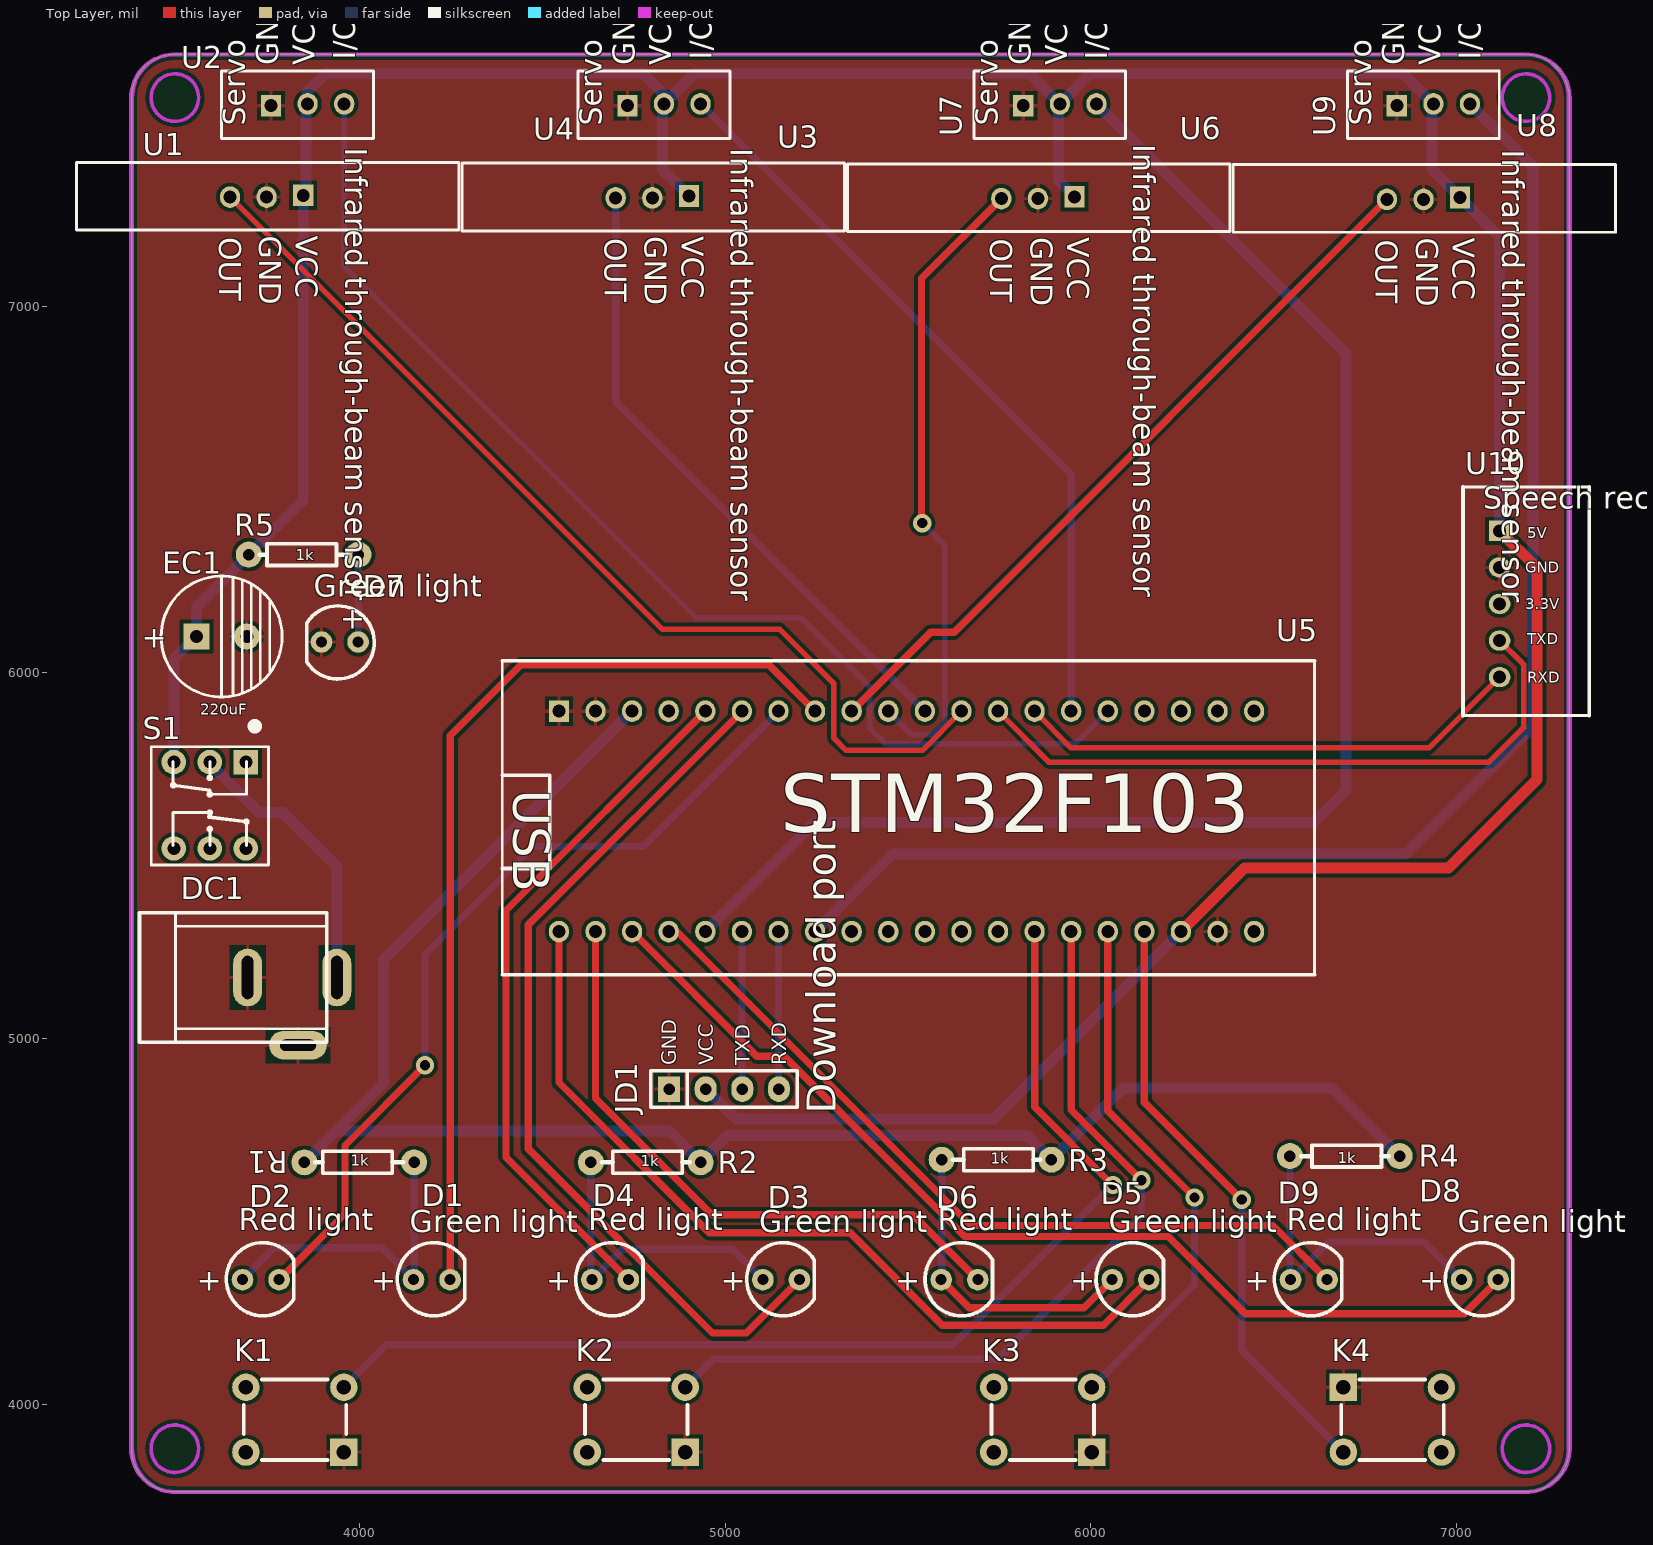
[diagram p0: Top Layer view]
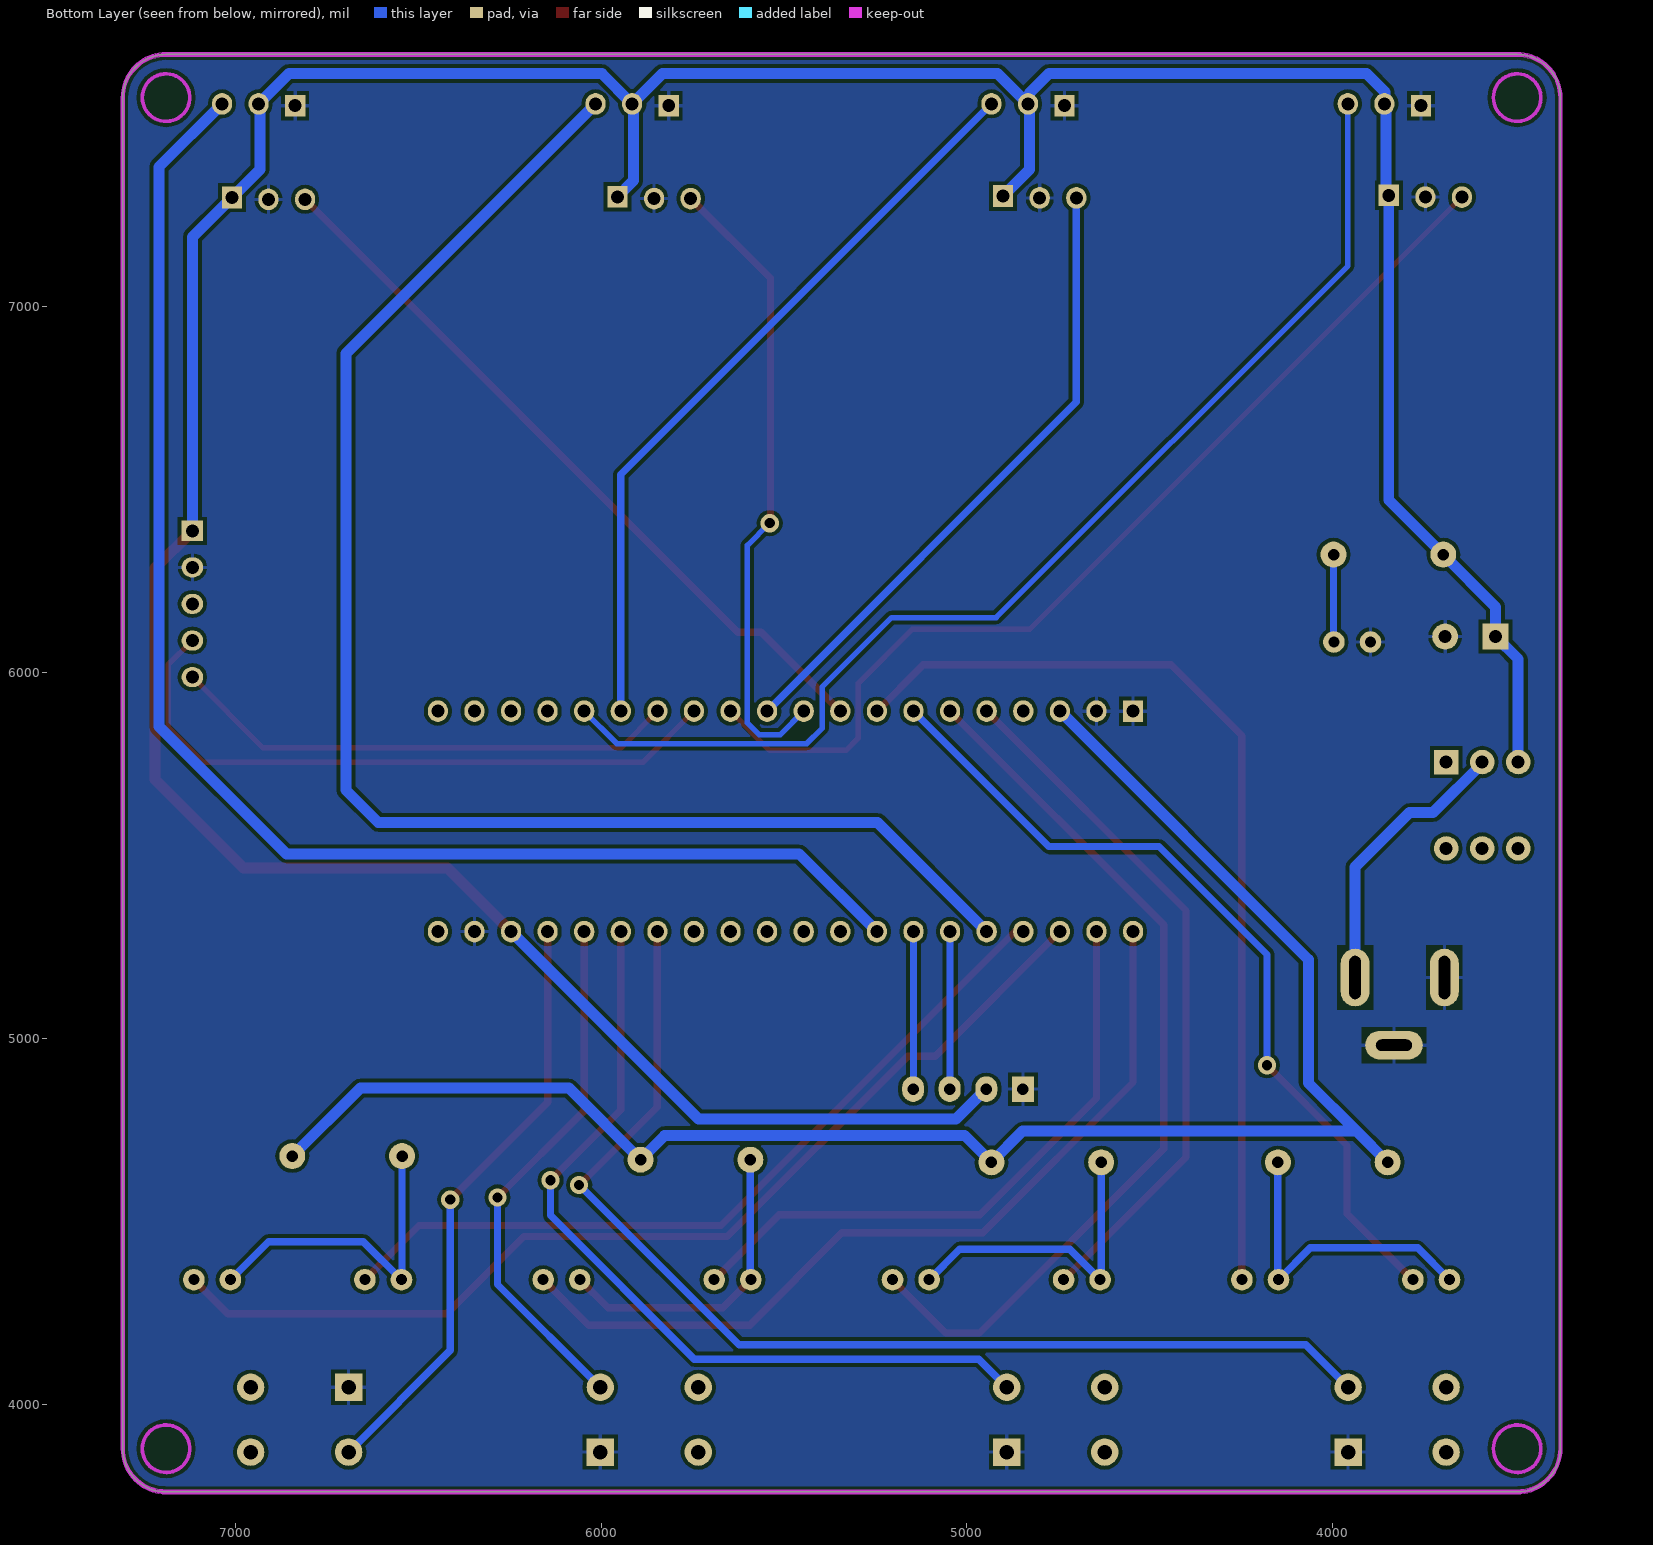
[diagram p1: Bottom Layer view, seen from below]
# Altium PCB MISC49886.pcbdoc
Units mil, origin at the board's own origin, x right, y up, seen from the top; angles counter-clockwise.
Board outline 3929.13 x 3929.13 mil, 2 copper layers (Top Layer, Bottom Layer); 32 components, 43 nets, 128 pads, 6 vias.

## Layer stack, top to bottom (the 12.6 mil dielectric is the usual default, probably not edited)
Top Solder Mask Layer: solder mask 1.4, FR-4, Dk 4.8
Top Layer: signal copper 1.4
Substrate1: surface 12.6, FR-4, Dk 4.8
Bottom Layer: signal copper 1.4
Bottom Solder Mask Layer: solder mask 1.4, FR-4, Dk 4.8

## Board outline
3378,7572.02 3378,3879.11 ccw(c3496.11,3879.11) 3496.11,3761 7189.02,3761 ccw(c7189.02,3879.11) 7307.13,3879.11 7307.13,7572.02 ccw(c7189.02,7572.02) 7189.02,7690.13 3496.11,7690.13 ccw(c3496.11,7572.02)

## Design rules (kind name [scope] priority, off if disabled: settings)
BoardOutlineClearance Clearance_1 [All] p2: genericclearance=10 ignorepadtopadclearanceinfootprint=FALSE except(0: Arc-SplitContinuation Track-SplitContinuation SMDPad-SplitContinuation THPad-SplitContinuation Via-SplitContinuation Fill-SplitContinuation Region-SplitContinuation Poly-SplitContinuation Text-SplitContinuation Hole-SplitContinuation; 6: SMDPad-CutoutEdge THPad-CutoutEdge Via-CutoutEdge Fill-CutoutEdge Region-CutoutEdge Text-CutoutEdge; 6.9: Hole-CutoutEdge; 10: Arc-OutlineEdge Track-OutlineEdge SMDPad-OutlineEdge THPad-OutlineEdge Via-OutlineEdge Fill-OutlineEdge Region-OutlineEdge Poly-OutlineEdge Text-OutlineEdge Hole-OutlineEdge Poly-CutoutEdge; 11.8: Arc-CutoutEdge Track-CutoutEdge)
Clearance [All] p1: gap=10 ignorepadtopadclearanceinfootprint=FALSE
DiffPairsRouting [All] p1: maxlimit=10 minlimit=6 mostfreqgap=6 toplayer_minwidth=0 toplayer_prefwidth=0 toplayer_maxwidth=0 toplayer_mingap=10 toplayer_prefgap=10 toplayer_maxgap=10 bottomlayer_minwidth=0 bottomlayer_prefwidth=0 bottomlayer_maxwidth=0 bottomlayer_mingap=10 bottomlayer_prefgap=10 bottomlayer_maxgap=10 maxuncoupledlength=10
HoleToHoleClearance ComponentClearance [All] p1: gap=10 allowstackedmicrovias=TRUE
Length netLength [All] p1: minlimit=0 maxlimit=0
MatchedLengths netLengthTolerance [All] p1: tolerance=1000
PolygonConnect [All] p1: connectstyle=Relief reliefconductorwidth=10 reliefentries=4 polygonreliefangle="90 Angle" airgapwidth=10 via.connectstyle=Relief via.reliefconductorwidth=10 via.reliefentries=4 via.polygonreliefangle="90 Angle" via.airgapwidth=10
RoutingVias [All] p1: holewidth=28 width=50 viastyle="Through Hole" minholewidth=28 minwidth=50 maxholewidth=28 maxwidth=50
SolderMaskExpansion [All] p1: expansion=4 istentingtop=FALSE
Width [All] p1: maxlimit=10 minlimit=10 preferedwidth=10 toplayer_minwidth=10 toplayer_maxwidth=40 toplayer_prefwidth=20 bottomlayer_minwidth=10 bottomlayer_maxwidth=40 bottomlayer_prefwidth=20
2 further rules are at their usual default settings.

## Components (designator, comment, footprint, x,y, rotation, side; value= is the part's Value field where it differs from the comment)
D1 "LED" LED5-GRE 4198.43,4341 r0 top
D2 "LED" LED5-RED 3731,4341 r0 top
D3 "LED" LED5-GRE 5153.29,4341 r0 top
D4 "LED" LED5-RED 4685.86,4341 r0 top
D5 "LED" LED5-GRE 6108.14,4341 r0 top
D6 "LED" LED5-RED 5640.71,4341 r0 top
D7 "LED" LED5-GRE 3947,6084 r180 top
D8 "LED" LED5-GRE 7063,4341 r0 top
D9 "LED" LED5-RED 6595.57,4341 r0 top
DC1 "DC_Socket" DC-005 3939,5167 r180 top
EC1 "220uF" DIP-EC3.5X8X11.5 3555,6099 r0 top
JD1 "Download port" 下载口 5187,5082 r180 top
K1 "BUTTOM" DIP-6X6X5 3958,3869.83 r180 top
K2 "BUTTOM" DIP-6X6X5 4891,3869.83 r180 top
K3 "BUTTOM" DIP-6X6X5 6002,3869.83 r180 top
K4 "BUTTOM" DIP-6X6X5 6690,4047 r0 top
R1 "1k" AXIAL0.3-1k 4150,4662 r180 top
R2 "1K" AXIAL0.3-1k 4633,4662 r0 top
R3 "1k" AXIAL0.3-1k 5592,4669 r0 top
R4 "1k" AXIAL0.3-1k 6544,4679 r0 top
R5 "1k" AXIAL0.3-1k 3998,6323 r180 top
S1 "KFT DIP-8X8" "KFT DIP-8X8" 3430,5801 r270 top
U1 "JS" JS 3217,7400 r270 top
U2 "SG90" SG90 4149,7460 r90 top
U3 "JS" JS 4271,7398 r270 top
U4 "SG90" SG90 5123,7460 r90 top
U5 "STM32F103" STM32F103 4546,5895 r270 top
U6 "JS" JS 5325,7396 r270 top
U7 "SG90" SG90 6205,7460 r90 top
U8 "JS" JS 6379,7394 r270 top
U9 "SG90" SG90 7226,7460 r90 top
U10 "SNR8016" SNR8016 7012,5878 r0 top

## Footprints (in the part's own frame and the unit in brackets; to place one, negate y for a bottom-side part, rotate by r counter-clockwise, add the part's x,y. Pads: shape width x height; smd on the part's side, far side on the other; paste and mask are expansions set on the pad)
AXIAL0.3-1k [mm]
  round 1.8 hole 0.8: 1(0,0) 2(7.62,0)
  silkscreen extent 0.76,-0.76 6.86,0.76
DC-005 [mm]
  oval 2x4 hole 0.8 slot 3 at 90 deg: 1(0,0) 2(6.2,0)
  oval 4x2 hole 0.8 slot 2.5 at 0 deg: 3(2.7,4.7)
  silkscreen extent 0.72,-4.5 13.7,4.5
DIP-6X6X5 [mm]
  rect 1.9x1.9 hole 1: 1(0,0)
  round 1.9 hole 1: 2(0,-4.5) 3(6.8,-4.5) 4(6.8,0)
  silkscreen extent -0.16,-5.04 6.96,0.54
DIP-EC3.5X8X11.5 [mm]
  rect 1.8x1.8 hole 0.9: 1(0,0)
  round 1.8 hole 0.9: 2(3.5,0)
  silkscreen extent -2.45,-4.2 5.95,4.2
JS [mm]
  rect 1.5x1.4 hole 0.9: 1(2.413,16.002)
  oval 1.5x1.4 hole 0.9: 2(2.54,13.462) 3(2.54,10.922)
  silkscreen extent 0.13,0.25 4.83,26.8
"KFT DIP-8X8" [mm]
  rect 1.7x1.7 hole 0.9: 1(1.143,6.604)
  round 1.7 hole 0.9: 2(1.143,4.104) 3(1.143,1.604) 4(7.143,1.604) 5(7.143,4.104) 6(7.143,6.604)
  silkscreen extent -1.54,0.04 8.3,8.17
LED5-GRE [mm]
  round 1.5 hole 0.762: A(-1.27,0) K(1.27,0)
  silkscreen extent -2.39,-2.51 2.29,2.57
LED5-RED [mm]
  round 1.5 hole 0.762: A(-1.27,0) K(1.27,0)
  silkscreen extent -2.39,-2.51 2.29,2.57
SG90 [mm]
  rect 1.5x1.4 hole 0.9: 1(2.286,9.906)
  oval 1.5x1.4 hole 0.9: 2(2.413,7.366) 3(2.413,4.826)
  silkscreen extent 0,2.79 4.7,13.33
SNR8016 [mm]
  rect 1.5x1.4 hole 0.9: 1(2.667,12.954)
  oval 1.5x1.4 hole 0.9: 2(2.667,10.414) 3(2.667,7.874) 4(2.667,5.334) 5(2.667,2.794)
  silkscreen extent 0.13,0.13 8.89,16
STM32F103 [mm]
  rect 1.5x1.4 hole 0.9: 1(0,0)
  oval 1.5x1.4 hole 0.9: 2(0,2.54) 3(0,5.08) 4(0,7.62) 5(0,10.16) 6(0,12.7) 7(0,15.24) 8(0,17.78) 9(0,20.32) 10(0,22.86) 11(0,25.4) 12(0,27.94) 13(0,30.48) 14(0,33.02) 15(0,35.56) 16(0,38.1) 17(0,40.64) 18(0,43.18) 19(0,45.72) 20(0,48.26) 25(15.3,48.26) 26(15.3,45.72) 27(15.3,43.18) 28(15.3,40.64) 29(15.3,38.1) 30(15.3,35.56) 31(15.3,33.02) 32(15.3,30.48) 33(15.3,27.94) 34(15.3,25.4) 35(15.3,22.86) 36(15.3,20.32) 37(15.3,17.78) 38(15.3,15.24) 39(15.3,12.7) 40(15.3,10.16) 41(15.3,7.62) 42(15.3,5.08) 43(15.3,2.54) 44(15.3,0)
  silkscreen extent -3.5,-3.94 18.29,52.45
下载口 [mil]
  rect 60x70 hole 32: 1(340,220)
  oval 60x70 hole 32: 2(240,220) 3(140,220) 4(40,220)
  silkscreen extent -10,170 390,270

## Via types
v1: diameter 50, hole 28, Top Layer to Bottom Layer, 6 vias

## Nets (pads, with @x,y where several pads share a name; then routed paths per layer and width w, separated by ;. In a path a pad name is that pad's centre, name@x,y a point inside that pad or via, vN(x,y) a via of type N, cw(c..) or ccw(c..) an arc to the next point about the centre after c; other vN are vias at no path point)
GND: D7.K DC1.2 DC1.3 EC1.2 JD1.1 K1.1 K2.1 K3.1 K4.1 U1.2 U2.1 U3.2 U4.1 U5.1 U5.2 U5.26 U6.2 U7.1 U8.2 U9.1 U10.2
NetD1_A: D1.A D2.A R1.1 | length 858.9
  Bottom Layer w20: D2.A 3768,4428 4061.43,4428 D1.A ; D1.A@4150,4342.57 R1.1
NetD3_A: D3.A D4.A R2.1 | length 858.4
  Bottom Layer w20: R2.1 4633,4343.86 D4.A 4718.86,4424 5020.29,4424 D3.A
NetD5_A: D5.A D6.A R3.1 | length 859.8
  Top Layer w20: D6.A 5667.71,4264 5981.14,4264 D5.A
  Bottom Layer w20: D6.A 5592,4342.29 R3.1
NetD7_A: D7.A R5.1 | length 238
  Bottom Layer w20: D7.A@3998,6085 R5.1
NetD8_A: D8.A D9.A R4.1 | length 890
  Bottom Layer w20: D9.A@6544,4342.57 R4.1 ; D9.A 6649.57,4445 6909,4445 D8.A
NetDC1_1: DC1.1 S1.2 | length 770.6
  Bottom Layer w30: S1.2 3591.57,5752.14 3725.72,5618 3790,5618 3939,5469 DC1.1
PA0: U2.3 U5.16 | length 3174
  Bottom Layer w15: U2.3 3959,7112 4920,6151 5206,6151 5396,5961 5396,5848 5438,5806 5957,5806 U5.16
PA1: U4.3 U5.15 | length 2079.6
  Bottom Layer w20: U4.3 5946,6542 U5.15
PA2: U5.14 U10.5 | length 1392.4
  Top Layer w15: U5.14 5946,5795 6924,5795 U10.5
PA3: U5.13 U10.4 | length 1799.1
  Top Layer w15: U5.13 5886,5755 7087,5755 7183,5851 7183,6022 U10.4
PA4: U1.3 U5.12 | length 2756.9
  Top Layer w15: U1.3 4828,6119 5149,6119 5297,5971 5297,5822 5331,5788 5539,5788 U5.12
PA5: U3.3 U5.11 | length 1753
  Bottom Layer w20: U3.3 4701,6740 U5.11
PA6: U5.10 U6.3 | length 1744.3
  Top Layer w20: v1@5537,6407 5537,7078 U6.3
  Bottom Layer w15: U5.10 5510,5831 5568,5831 5600,5863 5600,6348 v1(5539,6409)
PA7: U5.9 U8.3 | length 2042.5
  Top Layer w20: U5.9 5562,6111 5626,6111 U8.3
PA8: U5.40 U7.3 | length 4069.5
  Bottom Layer w30: U5.40 5244.36,5591 6609,5591 6697,5679 6697,6873 U7.3
PA9: JD1.3 U5.39 | length 429.6
  Bottom Layer w20: JD1.3@5046,4863 U5.39
PA10: JD1.4 U5.38 | length 429.6
  Bottom Layer w20: JD1.4@5146,4863 U5.38
PA11: U5.37 U9.3 | length 3967.4
  Bottom Layer w30: U5.37 5458.36,5505 6860,5505 7208,5853 7208,7383 U9.3
PA12: U5.36
PA15: U5.35
PB0: D1.K U5.8 | length 2617.8
  Top Layer w20: D1.K 4248.43,5828.43 4442,6022 5119,6022 U5.8
PB1: D2.K U5.7 | length 2295.7
  Top Layer w20: D2.K 3961,4521 3961,4708 v1(4180,4927)
  Bottom Layer w20: v1(4180,4927) 4180,5230 4475,5525 4776,5525 U5.7
PB3: U5.34
PB4: U5.33
PB5: U5.32
PB6: K1.2 U5.31 | length 3102
  Top Layer w20: U5.31 5846,4813 v1@6052,4607
  Bottom Layer w20: K1.2 4074,4163 5623,4163 v1(6060,4600)
PB7: K2.2 U5.30 | length 2296.8
  Top Layer w20: U5.30 5946,4805 v1(6138,4613)
  Bottom Layer w20: K2.2 4968,4124 5745,4124 6138,4517 v1(6138,4613)
PB8: K3.2 U5.29 | length 1460.2
  Top Layer w20: U5.29 6046,4803 v1(6283,4566)
  Bottom Layer w20: K3.2 6283,4328 v1(6283,4566)
PB9: K4.2 U5.28 | length 1648.1
  Top Layer w20: U5.28 6146,4826 v1(6412,4560)
  Bottom Layer w20: v1(6412,4560) 6412,4147.83 K4.2
PB10: D3.K U5.6 | length 2448.2
  Top Layer w20: U5.6 4462,5311 4462,4699 4965.71,4195.29 5057.57,4195.29 D3.K
PB11: D4.K U5.5 | length 1918.4
  Top Layer w20: D4.K 4401,4675.86 4401,5350 U5.5
PB12: D5.K U5.44 | length 2350.8
  Top Layer w20: U5.44 4546,4880 4957,4469 5342,4469 5594,4217 6034.14,4217 D5.K
PB13: D6.K U5.43 | length 1705.8
  Top Layer w20: U5.43 4646,4837 4964,4519 5512.71,4519 D6.K
PB14: D8.K U5.42 | length 2838.2
  Top Layer w20: U5.42 5086.64,4952 5162,4952 5655,4459 6211,4459 6422,4248 7020,4248 D8.K
PB15: D9.K U5.41 | length 2193.8
  Top Layer w20: U5.41 4868.36,5292.64 5672,4489 6497.57,4489 D9.K
PC13: U5.19
PC14: U5.18
PC15: U5.17
R: U5.4
VB: U5.20
VCC: EC1.1 JD1.2 R5.2 S1.3 U1.1 U2.2 U3.1 U4.2 U5.27 U6.1 U7.2 U8.1 U9.2 U10.1 | length 10465.3
  Top Layer w30: U5.27 6419.36,5466 6977,5466 7219,5708 7219,6286 U10.1
  Bottom Layer w30: S1.3 3493.15,6037.15 EC1.1 3555,6180 R5.2 3847,6472 U1.1 3855,7313 3855,7564 3857,7566 3857,7587 3908,7638 4776,7638 4829,7585 4829,7375 U3.1 ; U4.2 4916,7638 5832,7638 U7.2 5998,7638 6853,7638 U9.2 ; JD1.2@4956,4854 5030,4780 5733.36,4780 U5.27 ; U7.2@5911,7555 5911,7345 U6.1 ; U9.2@6932,7555 6932,7376 U8.1 7117,7191 U10.1
VCC_3V3: R1.2 R2.2 R3.2 R4.2 U5.3 | length 4764.1
  Bottom Layer w30: R1.2 3935,4747 ; U5.3 4067,5216 4067,4879 3935,4747 ; R4.2 6658,4865 6088,4865 R3.2 5826,4735 5006,4735 R2.2 4848,4747 3935,4747
pads on no net: K1.3 K1.4 K2.3 K2.4 K3.3 K3.4 K4.3 K4.4 S1.1 S1.4 S1.5 S1.6 U5.25 U10.3

## Polygon pours and split planes (outlines as drawn)
GND on Bottom Layer (solid, remove dead copper, pour order 6): 3000,7913 3018,7931 7474,7931 7474,3375 7367,3268 7161,3474 3053,3474
GND on Top Layer (solid, remove dead copper, pour order 8): 3089,7743 7582,7743 7456,7617 7456,3000 3715,3000 3250,3465

## Keep-outs
Board Outline Layer:
  region: 7312.13,3879.11 7311.75,3869.45 7310.62,3859.85 7308.73,3850.37 7306.11,3841.07 7302.76,3832 7298.72,3823.22 7293.99,3814.79 7288.62,3806.75 7282.64,3799.16 7276.08,3792.06 7268.98,3785.5 7261.39,3779.51 7253.35,3774.14 7244.91,3769.42 7236.14,3765.37 7227.07,3762.03 7217.76,3759.4 7208.28,3757.52 7198.68,3756.38 7189.02,3756 7187.11,3756.38 7185.49,3757.46 7184.4,3759.09 7184.02,3761 7184.4,3762.91 7185.49,3764.54 7187.11,3765.62 7189.02,3766 7198.36,3766.39 7207.64,3767.54 7216.79,3769.46 7225.75,3772.13 7234.46,3775.53 7242.86,3779.63 7250.89,3784.42 7258.5,3789.85 7265.63,3795.89 7272.24,3802.5 7278.28,3809.64 7283.72,3817.24 7288.5,3825.28 7292.61,3833.67 7296.01,3842.38 7298.67,3851.34 7300.59,3860.49 7301.75,3869.77 7302.13,3879.11 7302.51,3881.02 7303.6,3882.65 7305.22,3883.73 7307.13,3884.11 7309.05,3883.73 7310.67,3882.65 7311.75,3881.02
  region: 7312.13,7572.02 7311.75,7570.11 7310.67,7568.49 7309.05,7567.4 7307.13,7567.02 7305.22,7567.4 7303.6,7568.49 7302.51,7570.11 7302.13,7572.02 7301.75,7581.36 7300.59,7590.64 7298.67,7599.79 7296.01,7608.75 7292.61,7617.46 7288.5,7625.86 7283.72,7633.89 7278.28,7641.5 7272.24,7648.63 7265.63,7655.24 7258.5,7661.28 7250.89,7666.72 7242.86,7671.5 7234.46,7675.61 7225.75,7679.01 7216.79,7681.67 7207.64,7683.59 7198.36,7684.75 7189.02,7685.13 7187.11,7685.51 7185.49,7686.6 7184.4,7688.22 7184.02,7690.13 7184.4,7692.05 7185.49,7693.67 7187.11,7694.75 7189.02,7695.13 7198.68,7694.75 7208.28,7693.62 7217.76,7691.73 7227.07,7689.11 7236.14,7685.76 7244.91,7681.72 7253.35,7676.99 7261.39,7671.62 7268.98,7665.64 7276.08,7659.08 7282.64,7651.98 7288.62,7644.39 7293.99,7636.35 7298.72,7627.91 7302.76,7619.14 7306.11,7610.07 7308.73,7600.76 7310.62,7591.28 7311.75,7581.68
  region: 3383,7572.02 3382.62,7570.11 3381.54,7568.49 3379.91,7567.4 3378,7567.02 3376.09,7567.4 3374.46,7568.49 3373.38,7570.11 3373,7572.02 3373.38,7581.68 3374.52,7591.28 3376.4,7600.76 3379.03,7610.07 3382.37,7619.14 3386.42,7627.91 3391.14,7636.35 3396.51,7644.39 3402.5,7651.98 3409.06,7659.08 3416.16,7665.64 3423.75,7671.62 3431.79,7676.99 3440.22,7681.72 3449,7685.76 3458.07,7689.11 3467.37,7691.73 3476.85,7693.62 3486.45,7694.75 3496.11,7695.13 3498.02,7694.75 3499.65,7693.67 3500.73,7692.05 3501.11,7690.13 3500.73,7688.22 3499.65,7686.6 3498.02,7685.51 3496.11,7685.13 3486.77,7684.75 3477.49,7683.59 3468.34,7681.67 3459.38,7679.01 3450.67,7675.61 3442.28,7671.5 3434.24,7666.72 3426.64,7661.28 3419.5,7655.24 3412.89,7648.63 3406.85,7641.5 3401.42,7633.89 3396.63,7625.86 3392.53,7617.46 3389.13,7608.75 3386.46,7599.79 3384.54,7590.64 3383.39,7581.36
  region: 3496.11,3756 3486.45,3756.38 3476.85,3757.52 3467.37,3759.4 3458.07,3762.03 3449,3765.37 3440.22,3769.42 3431.79,3774.14 3423.75,3779.51 3416.16,3785.5 3409.06,3792.06 3402.5,3799.16 3396.51,3806.75 3391.14,3814.79 3386.42,3823.22 3382.37,3832 3379.03,3841.07 3376.4,3850.37 3374.52,3859.85 3373.38,3869.45 3373,3879.11 3373.38,3881.02 3374.46,3882.65 3376.09,3883.73 3378,3884.11 3379.91,3883.73 3381.54,3882.65 3382.62,3881.02 3383,3879.11 3383.39,3869.77 3384.54,3860.49 3386.46,3851.34 3389.13,3842.38 3392.53,3833.67 3396.63,3825.28 3401.42,3817.24 3406.85,3809.64 3412.89,3802.5 3419.5,3795.89 3426.64,3789.85 3434.24,3784.42 3442.28,3779.63 3450.67,3775.53 3459.38,3772.13 3468.34,3769.46 3477.49,3767.54 3486.77,3766.39 3496.11,3766 3498.02,3765.62 3499.65,3764.54 3500.73,3762.91 3501.11,3761 3500.73,3759.09 3499.65,3757.46 3498.02,3756.38
  region: 3561.07,3879.11 cw(c3496.11,3879.11) 3431.15,3879.11 cw(c3496.11,3879.11)
  circle w10: c3496.11,3879.11 r64.96
  region: 7253.98,3879.11 cw(c7189.02,3879.11) 7124.06,3879.11 cw(c7189.02,3879.11)
  circle w10: c7189.02,3879.11 r64.96
  region: 7253.98,7572.02 cw(c7189.02,7572.02) 7124.06,7572.02 cw(c7189.02,7572.02)
  circle w10: c7189.02,7572.02 r64.96
  region: 3561.07,7572.02 cw(c3496.11,7572.02) 3431.15,7572.02 cw(c3496.11,7572.02)
  circle w10: c3496.11,7572.02 r64.96
  region: 7194.02,3761 7193.64,3759.09 7192.56,3757.46 7190.94,3756.38 7189.02,3756 3496.11,3756 3494.2,3756.38 3492.57,3757.46 3491.49,3759.09 3491.11,3761 3491.49,3762.91 3492.57,3764.54 3494.2,3765.62 3496.11,3766 7189.02,3766 7190.94,3765.62 7192.56,3764.54 7193.64,3762.91
  region: 7194.02,7690.13 7193.64,7688.22 7192.56,7686.6 7190.94,7685.51 7189.02,7685.13 3496.11,7685.13 3494.2,7685.51 3492.57,7686.6 3491.49,7688.22 3491.11,7690.13 3491.49,7692.05 3492.57,7693.67 3494.2,7694.75 3496.11,7695.13 7189.02,7695.13 7190.94,7694.75 7192.56,7693.67 7193.64,7692.05
  region: 3378,3874.11 3376.09,3874.49 3374.46,3875.57 3373.38,3877.2 3373,3879.11 3373,7572.02 3373.38,7573.94 3374.46,7575.56 3376.09,7576.64 3378,7577.02 3379.91,7576.64 3381.54,7575.56 3382.62,7573.94 3383,7572.02 3383,3879.11 3382.62,3877.2 3381.54,3875.57 3379.91,3874.49
  region: 7307.13,3874.11 7305.22,3874.49 7303.6,3875.57 7302.51,3877.2 7302.13,3879.11 7302.13,7572.02 7302.51,7573.94 7303.6,7575.56 7305.22,7576.64 7307.13,7577.02 7309.05,7576.64 7310.67,7575.56 7311.75,7573.94 7312.13,7572.02 7312.13,3879.11 7311.75,3877.2 7310.67,3875.57 7309.05,3874.49
  lines w10: 3378,3879.11 ccw(c3496.11,3879.11) 3496.11,3761 7189.02,3761 ccw(c7189.02,3879.11) 7307.13,3879.11 7307.13,7572.02 ccw(c7189.02,7572.02) 7189.02,7690.13 3496.11,7690.13 ccw(c3496.11,7572.02) 3378,7572.02 3378,3879.11